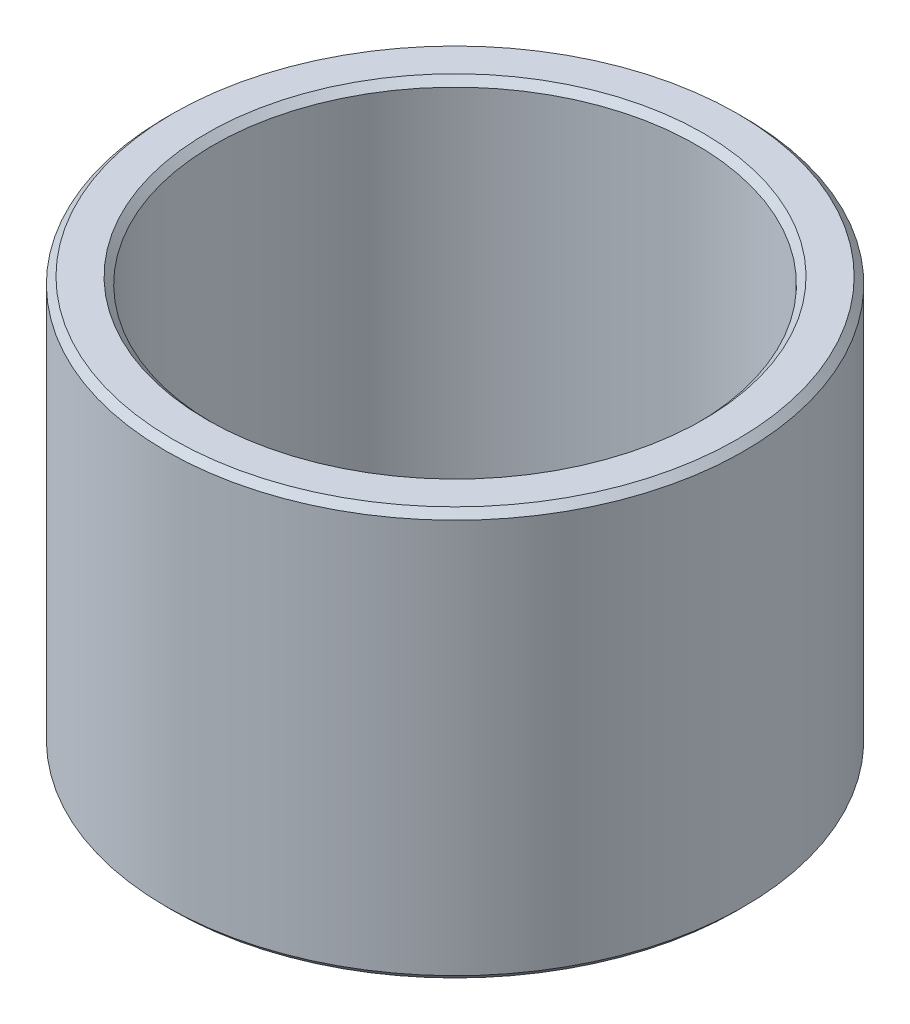
SolidWorks part; units mm, degrees
material "Q235B"
ref_plane "Front Plane" through (0, 0, 0) normal (0, 0, 1) x (1, 0, 0)
ref_plane "Top Plane" through (0, 0, 0) normal (0, 1, 0) x (1, 0, 0)
ref_plane "Right Plane" through (0, 0, 0) normal (1, 0, 0) x (0, 0, -1)
sketch "Sketch1" plane through (0, 0, 0) normal (0, 1, 0) x (1, 0, 0)
  circle A0 centre (0, 0) radius 35.5
  circle A1 centre (0, 0) radius 42.5
  dimension "D1" = 71
  dimension "D2" = 85
extrude "Boss-Extrude1" add sketch "Sketch1" along normal blind 60
chamfer "Chamfer2" distance 1 angle 45 4 edges at (0, 0, 35.5) (0, 60, 35.5) (0, 0, 42.5) (0, 60, 42.5)
